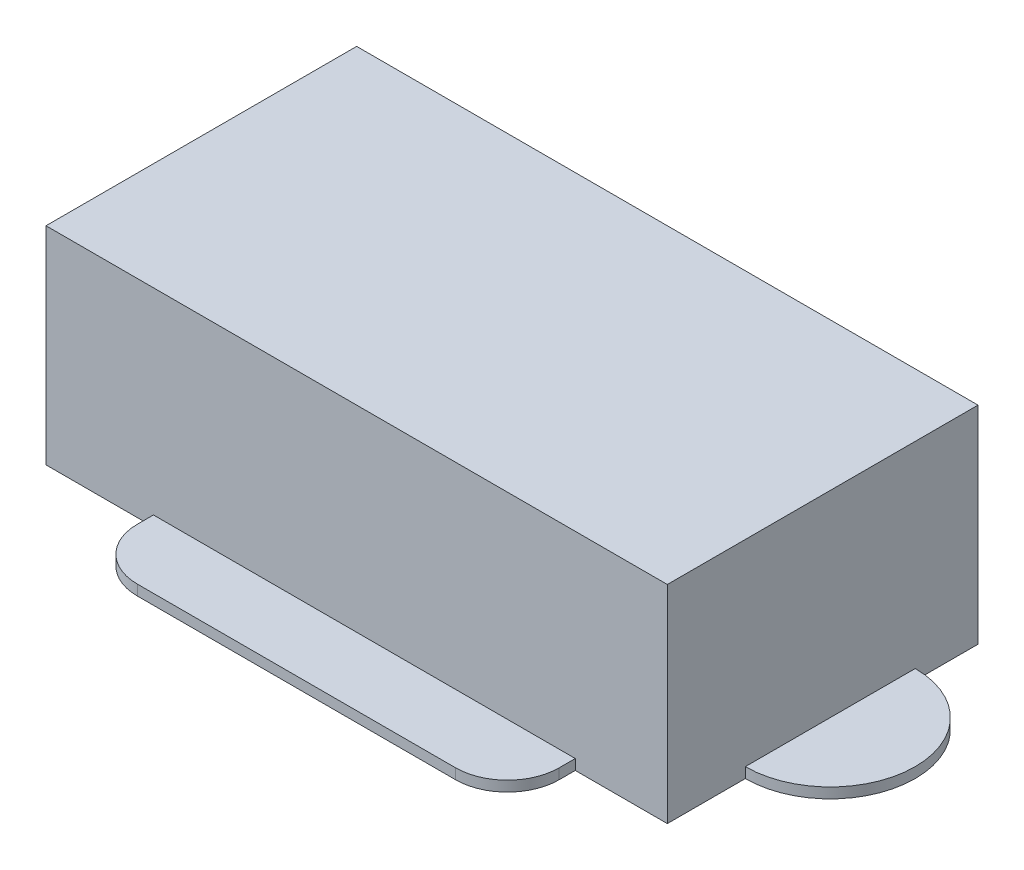
from build123d import *

# Parameters (mm, degrees)
SKETCH1_W           = 60
SKETCH1_H           = 30
BOSS_EXTRUDE1_DEPTH = 20
SKETCH2_W           = 37.506064646
SKETCH2_H           = 6.251724505
BOSS_EXTRUDE2_DEPTH = 5
BOSS_EXTRUDE3_DEPTH = 1


with BuildPart() as part:
    # Sketch1 → Boss-Extrude1 (new body)
    with BuildSketch(Plane(origin=(0, 0, 0), x_dir=(1, 0, 0), z_dir=(0, 1, 0))):
        Rectangle(SKETCH1_W, SKETCH1_H)
    extrude(amount=BOSS_EXTRUDE1_DEPTH)

    # Sketch2 → Boss-Extrude2 (add)
    with BuildSketch(Plane(origin=(0, 0, -15), x_dir=(-1, 0, 0), z_dir=(0, 0, -1))):
        with Locations((0, 9.939278845)):
            Rectangle(SKETCH2_W, SKETCH2_H)
    extrude(amount=BOSS_EXTRUDE2_DEPTH)

    # Sketch3 → Boss-Extrude3 (add)
    with BuildSketch(Plane.XZ):
        with BuildLine():
            Line((-30, 7.472956379), (-30, -8.939791774))
            ThreePointArc((-30, -8.939791774), (-38.206374076, -0.733417697), (-30, 7.472956379))
        make_face()
        with BuildLine():
            Line((30, 7.472956379), (30, -8.939791774))
            ThreePointArc((30, -8.939791774), (38.206374076, -0.733417697), (30, 7.472956379))
        make_face()
        with BuildLine():
            Line((-19.626363832, 15), (21.109917151, 15))
            Line((21.109917151, 15), (21.109917151, 16.556070662))
            ThreePointArc((21.109917151, 16.556070662), (19.645451057, 20.091604568), (16.109917151, 21.556070662))
            Line((16.109917151, 21.556070662), (-14.626363832, 21.556070662))
            ThreePointArc((-14.626363832, 21.556070662), (-18.161897738, 20.091604568), (-19.626363832, 16.556070662))
            Line((-19.626363832, 16.556070662), (-19.626363832, 15))
        make_face()
    extrude(amount=-BOSS_EXTRUDE3_DEPTH)


solid = part.part
